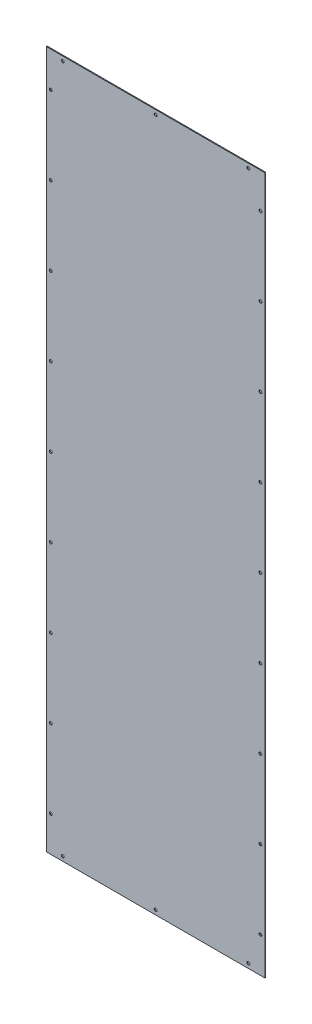
from build123d import *

# Parameters (mm, degrees)
SKETCH_1_W      = 494.5
SKETCH_1_H      = 1578
SKETCH_1_R      = 3.25
EXTRUDE_1_DEPTH = 2


with BuildPart() as part:
    # 草图1 → 凸台-拉伸1 (new body)
    with BuildSketch(Plane.XY):
        Rectangle(SKETCH_1_W, SKETCH_1_H)
        with Locations((-237.25, 0)):
            Circle(SKETCH_1_R, mode=Mode.SUBTRACT)
        with Locations((-237.25, -177.25)):
            Circle(SKETCH_1_R, mode=Mode.SUBTRACT)
        with Locations((-237.25, -354.5)):
            Circle(SKETCH_1_R, mode=Mode.SUBTRACT)
        with Locations((-237.25, -531.75)):
            Circle(SKETCH_1_R, mode=Mode.SUBTRACT)
        with Locations((-237.25, -709)):
            Circle(SKETCH_1_R, mode=Mode.SUBTRACT)
        with Locations((0, -779)):
            Circle(SKETCH_1_R, mode=Mode.SUBTRACT)
        with Locations(Location((0, 779, 0), (0, 0, 180))):
            Circle(SKETCH_1_R, mode=Mode.SUBTRACT)
        with Locations(Location((-237.25, 709, 0), (0, 0, 180))):
            Circle(SKETCH_1_R, mode=Mode.SUBTRACT)
        with Locations(Location((-237.25, 531.75, 0), (0, 0, 180))):
            Circle(SKETCH_1_R, mode=Mode.SUBTRACT)
        with Locations(Location((-237.25, 354.5, 0), (0, 0, 180))):
            Circle(SKETCH_1_R, mode=Mode.SUBTRACT)
        with Locations(Location((-237.25, 177.25, 0), (0, 0, 180))):
            Circle(SKETCH_1_R, mode=Mode.SUBTRACT)
        with Locations((237.25, 177.25)):
            Circle(SKETCH_1_R, mode=Mode.SUBTRACT)
        with Locations((237.25, 354.5)):
            Circle(SKETCH_1_R, mode=Mode.SUBTRACT)
        with Locations((237.25, 531.75)):
            Circle(SKETCH_1_R, mode=Mode.SUBTRACT)
        with Locations((237.25, 709)):
            Circle(SKETCH_1_R, mode=Mode.SUBTRACT)
        with Locations(Location((237.25, -709, 0), (0, 0, 180))):
            Circle(SKETCH_1_R, mode=Mode.SUBTRACT)
        with Locations(Location((237.25, -531.75, 0), (0, 0, 180))):
            Circle(SKETCH_1_R, mode=Mode.SUBTRACT)
        with Locations(Location((237.25, -354.5, 0), (0, 0, 180))):
            Circle(SKETCH_1_R, mode=Mode.SUBTRACT)
        with Locations(Location((237.25, -177.25, 0), (0, 0, 180))):
            Circle(SKETCH_1_R, mode=Mode.SUBTRACT)
        with Locations(Location((237.25, 0, 0), (0, 0, 180))):
            Circle(SKETCH_1_R, mode=Mode.SUBTRACT)
        with Locations((-210, 779)):
            Circle(SKETCH_1_R, mode=Mode.SUBTRACT)
        with Locations((210, 779)):
            Circle(SKETCH_1_R, mode=Mode.SUBTRACT)
        with Locations(Location((210, -779, 0), (0, 0, 180))):
            Circle(SKETCH_1_R, mode=Mode.SUBTRACT)
        with Locations(Location((-210, -779, 0), (0, 0, 180))):
            Circle(SKETCH_1_R, mode=Mode.SUBTRACT)
    extrude(amount=EXTRUDE_1_DEPTH)


solid = part.part
